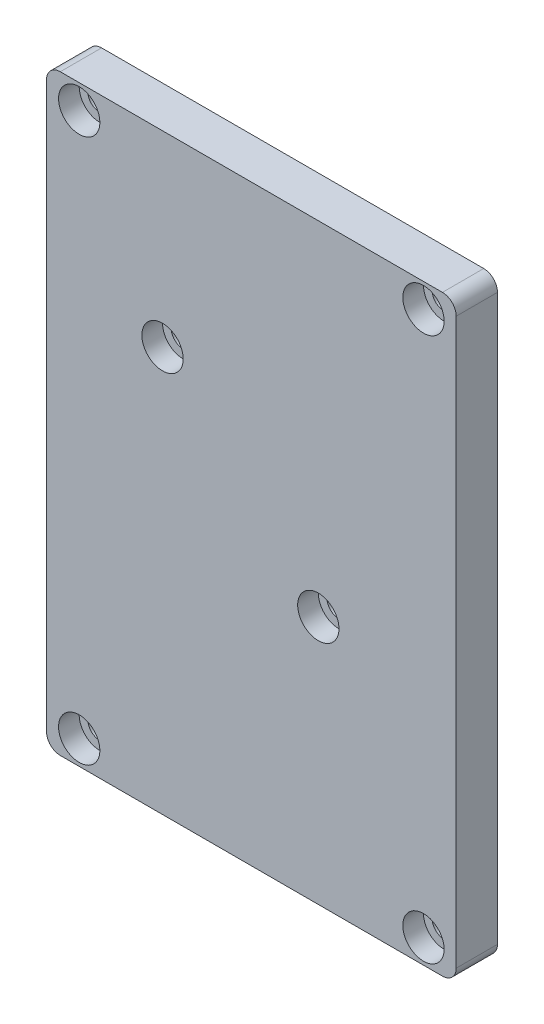
SolidWorks part; units mm, degrees
material "6061 合金"
ref_plane "前视基准面" through (0, 0, 0) normal (0, 0, 1) x (1, 0, 0)
ref_plane "上视基准面" through (0, 0, 0) normal (0, 1, 0) x (1, 0, 0)
ref_plane "右视基准面" through (0, 0, 0) normal (1, 0, 0) x (0, 0, -1)
sketch "草图1" plane through (0, 0, 0) normal (0, 0, 1) x (1, 0, 0)
  line L1 (-29.75, 43) -> (29.75, 43)
  line L2 (-29.75, 43) -> (-29.75, -43)
  line L3 (-29.75, -43) -> (29.75, -43)
  line L4 (29.75, 43) -> (29.75, -43)
  line L5 (-29.75, 43) -> (29.75, -43) construction
  line L6 (-29.75, -43) -> (29.75, 43) construction
  point P0 (0, 0)
  dimension "D1" = 86
  dimension "D2" = 59.5
extrude "凸台-拉伸1" add sketch "草图1" along normal blind 6
sketch "草图2" plane through (0, 0, 6) normal (0, 0, 1) x (1, 0, 0)
  line L0 (-60.4346, 0) -> (40.7542, 0) construction
  line L1 (0, -50.246) -> (0, 47.1111) construction
  line L2 (-60.4346, -39.5) -> (40.7542, -39.5) construction
  line L3 (-60.4346, 39.5) -> (40.7542, 39.5) construction
  line L4 (25, -50.246) -> (25, 47.1111) construction
  line L5 (-25, -50.246) -> (-25, 47.1111) construction
  line L8 (-12.9, -50.246) -> (-12.9, 47.1111) construction
  line L9 (29.75, 15.8) -> (-29.75, 15.8)
  line L10 (29.75, 15.8) -> (-29.75, 15.8) construction
  line L11 (-12.9, 15.8) -> (9.7274, -6.8274) construction
  circle A0 centre (-25, -39.5) radius 1.75
  circle A1 centre (25, -39.5) radius 1.75
  circle A2 centre (25, 39.5) radius 1.75
  circle A3 centre (-25, 39.5) radius 1.75
  circle A4 centre (-12.9, 15.8) radius 1.75
  circle A5 centre (9.7274, -6.8274) radius 1.75
  dimension "D7" = 3.5
  dimension "D8" = 3.5
  dimension "D11" = 3.5
  dimension "D12" = 3.5
  dimension "D13" = 3.5
  dimension "D14" = 3.5
  dimension "D9" = 32
  dimension "D10" = 45
  dimension "D1" = 39.5
  dimension "D2" = 39.5
  dimension "D3" = 25
  dimension "D4" = 25
  dimension "D5" = 27.2
  dimension "D6" = 12.9
extrude "切除-拉伸1" cut sketch "草图2" against normal blind 6
sketch "草图3" plane through (0, 0, 6) normal (0, 0, 1) x (1, 0, 0)
  circle A0 centre (-25, 39.5) radius 3
  circle A1 centre (25, 39.5) radius 3
  circle A2 centre (-12.9, 15.8) radius 3
  circle A3 centre (9.7274, -6.8274) radius 3
  circle A4 centre (-25, -39.5) radius 3
  circle A5 centre (25, -39.5) radius 3
  dimension "D1" = 6
  dimension "D2" = 6
  dimension "D3" = 6
  dimension "D4" = 6
  dimension "D5" = 6
  dimension "D6" = 6
extrude "切除-拉伸2" cut sketch "草图3" against normal blind 3
fillet "圆角1" radius 2 4 edges at (-29.75, -43, 3) (29.75, -43, 3) (29.75, 43, 3) (-29.75, 43, 3)
